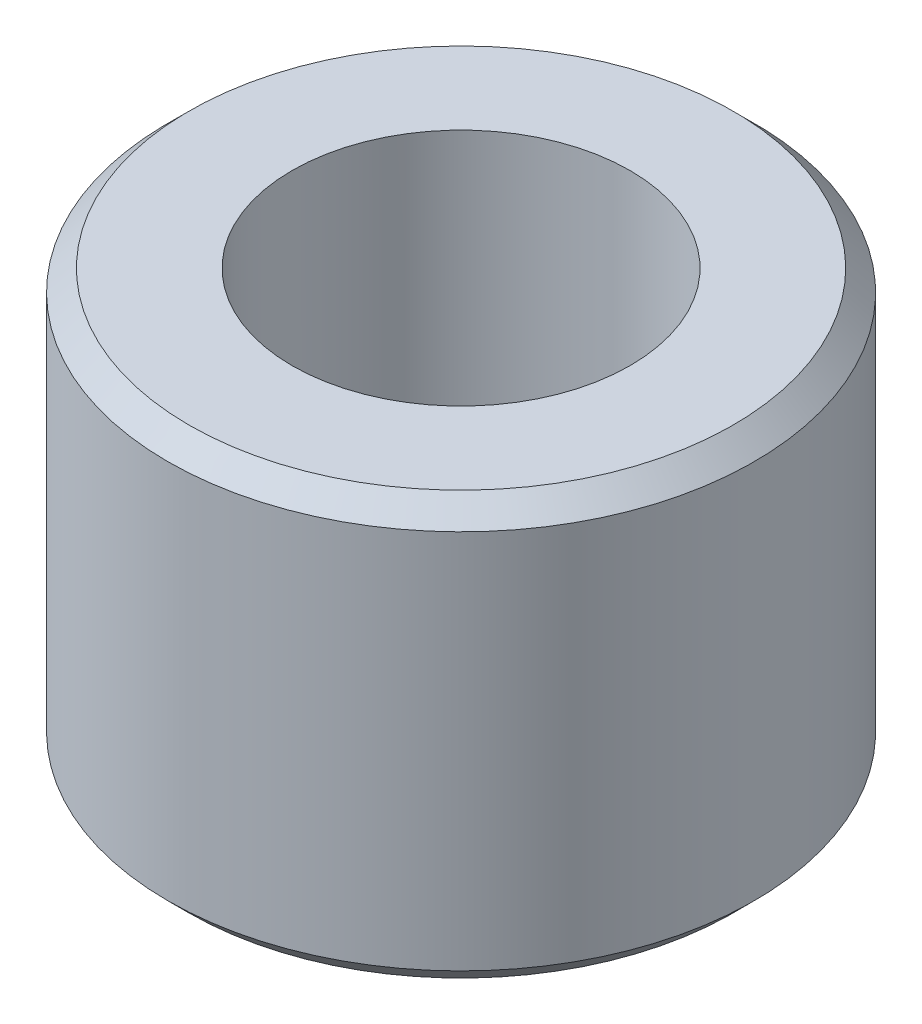
SolidWorks part; units mm, degrees
ref_plane "前视基准面" through (0, 0, 0) normal (0, 0, 1) x (1, 0, 0)
ref_plane "上视基准面" through (0, 0, 0) normal (0, 1, 0) x (1, 0, 0)
ref_plane "右视基准面" through (0, 0, 0) normal (1, 0, 0) x (0, 0, -1)
sketch "草图1" plane through (0, 0, 0) normal (0, 1, 0) x (1, 0, 0)
  circle A0 centre (0, 0) radius 16
  circle A1 centre (0, 0) radius 27.75
  dimension "D1" = 32
  dimension "D2" = 55.5
extrude "凸台-拉伸1" add sketch "草图1" along normal blind 40
chamfer "倒角1" distance 2 angle 45 2 edges at (0, 40, 27.75) (0, 0, 27.75)
sketch "草图2" plane through (0, 0, 0) normal (0, -1, 0) x (1, 0, 0)
  circle A0 centre (0, 0) radius 16
  circle A1 centre (0, 0) radius 7.5
  dimension "D1" = 15
extrude "凸台-拉伸2" add sketch "草图2" against normal blind 5
